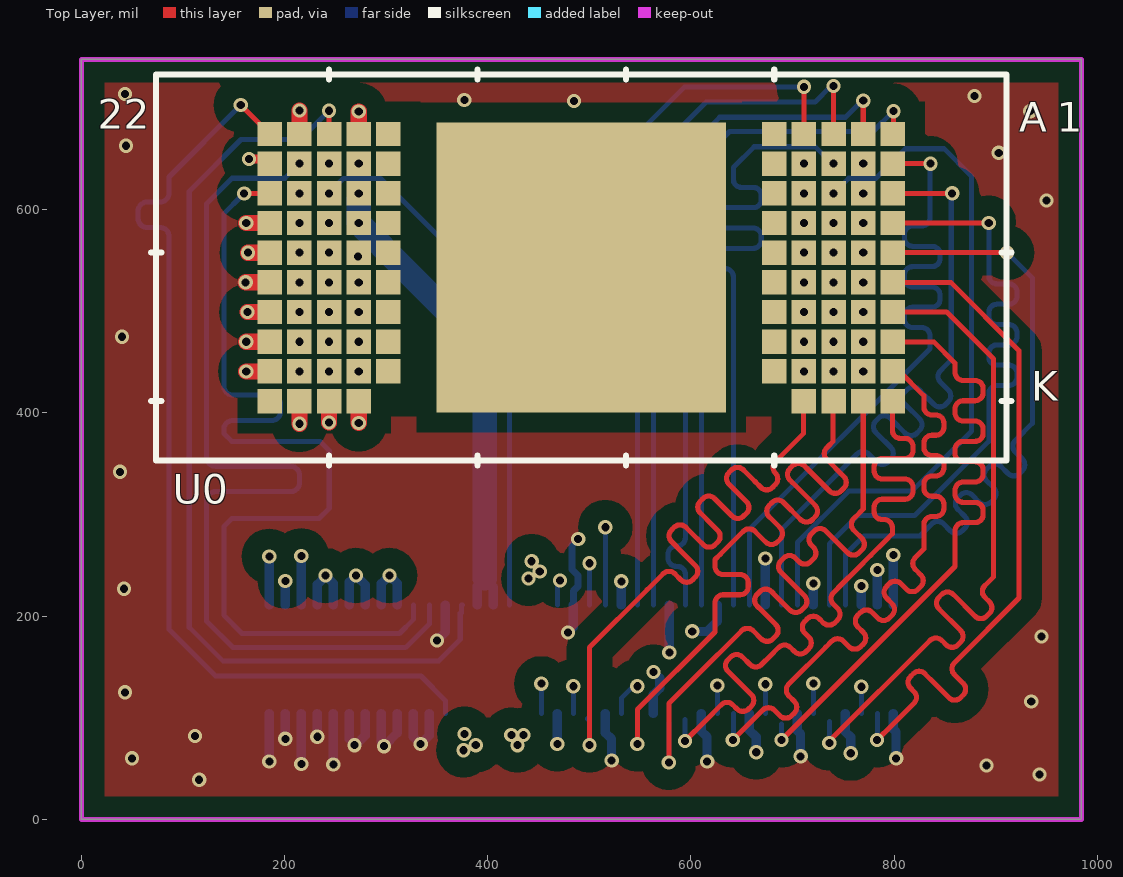
[diagram p0: Top Layer view]
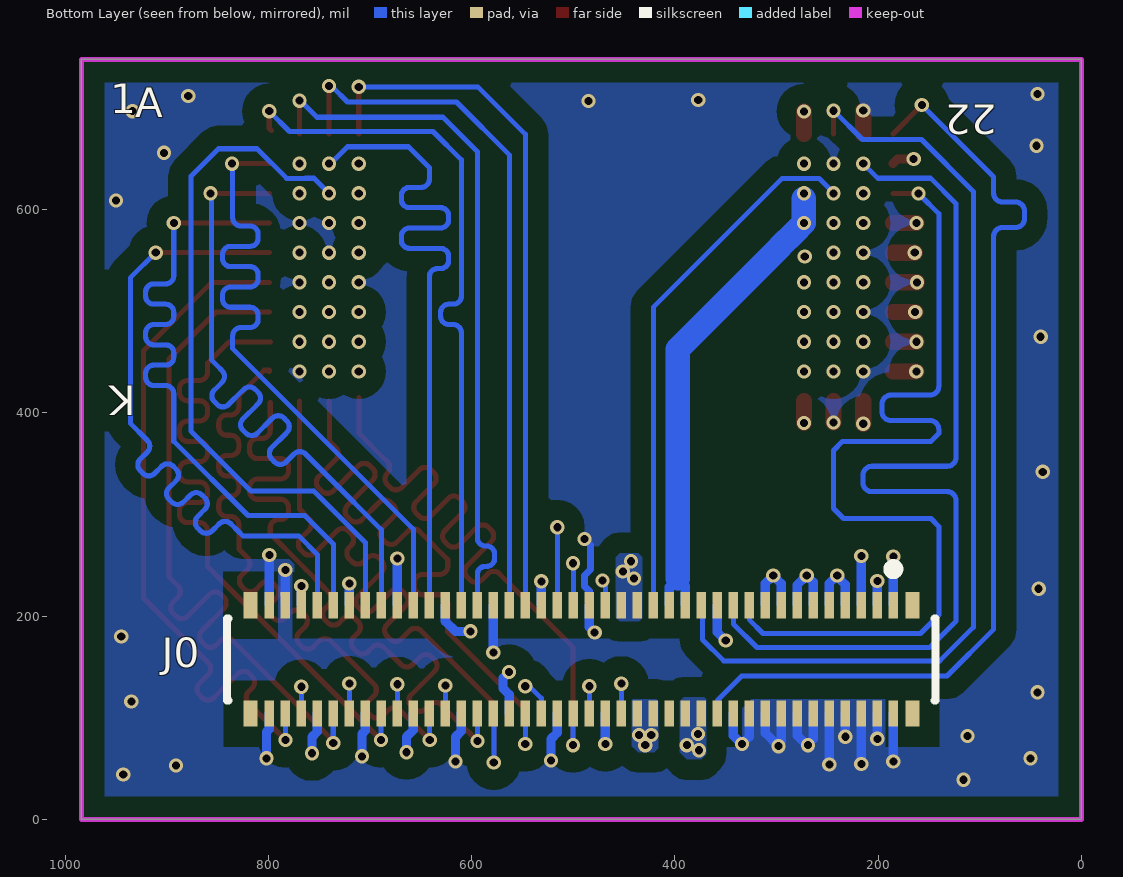
[diagram p1: Bottom Layer view, seen from below]
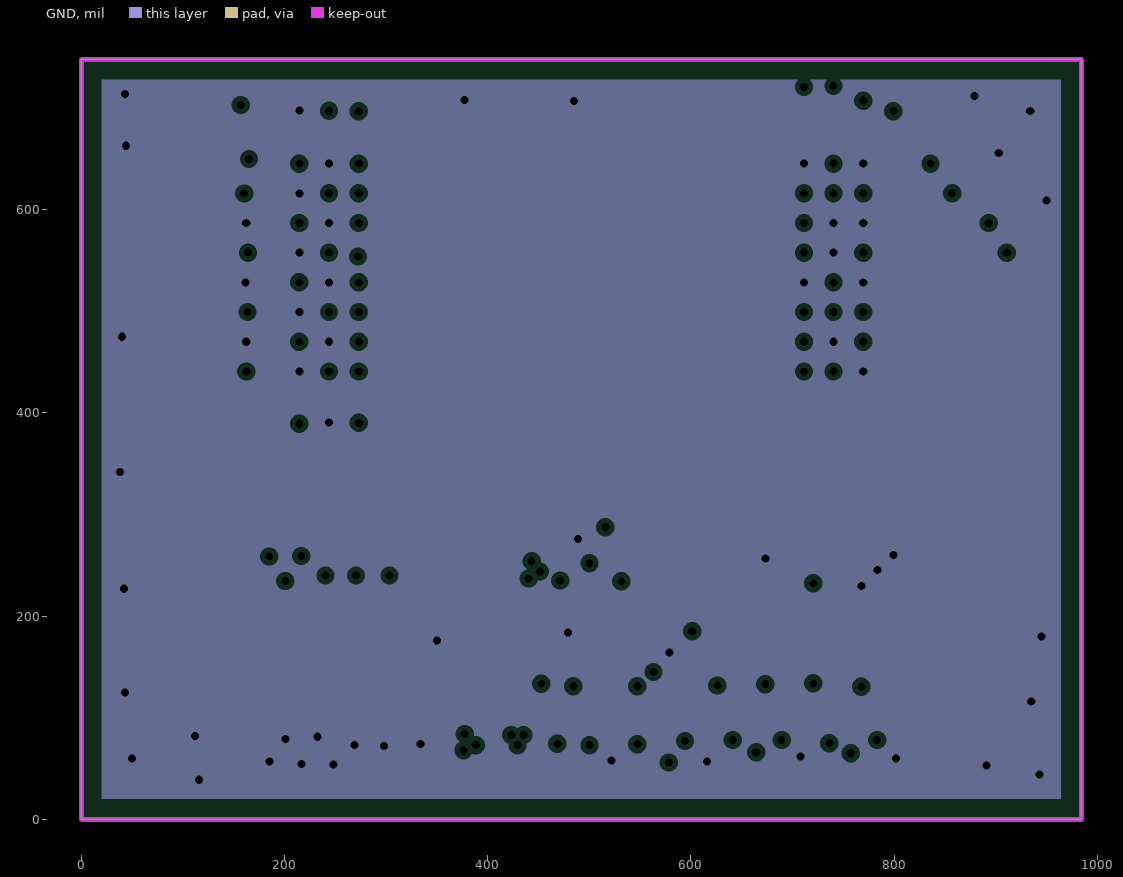
[diagram p2: GND, clearances drawn from the general rule]
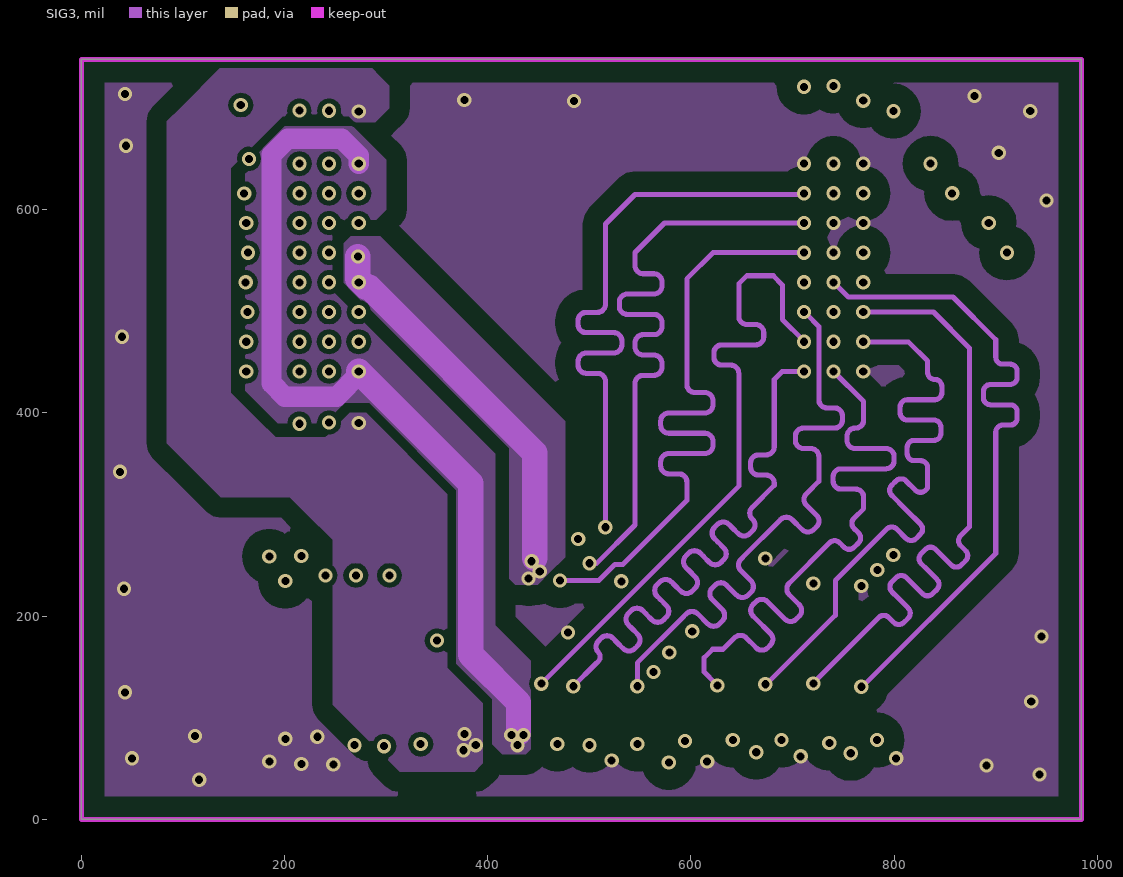
[diagram p3: SIG3]
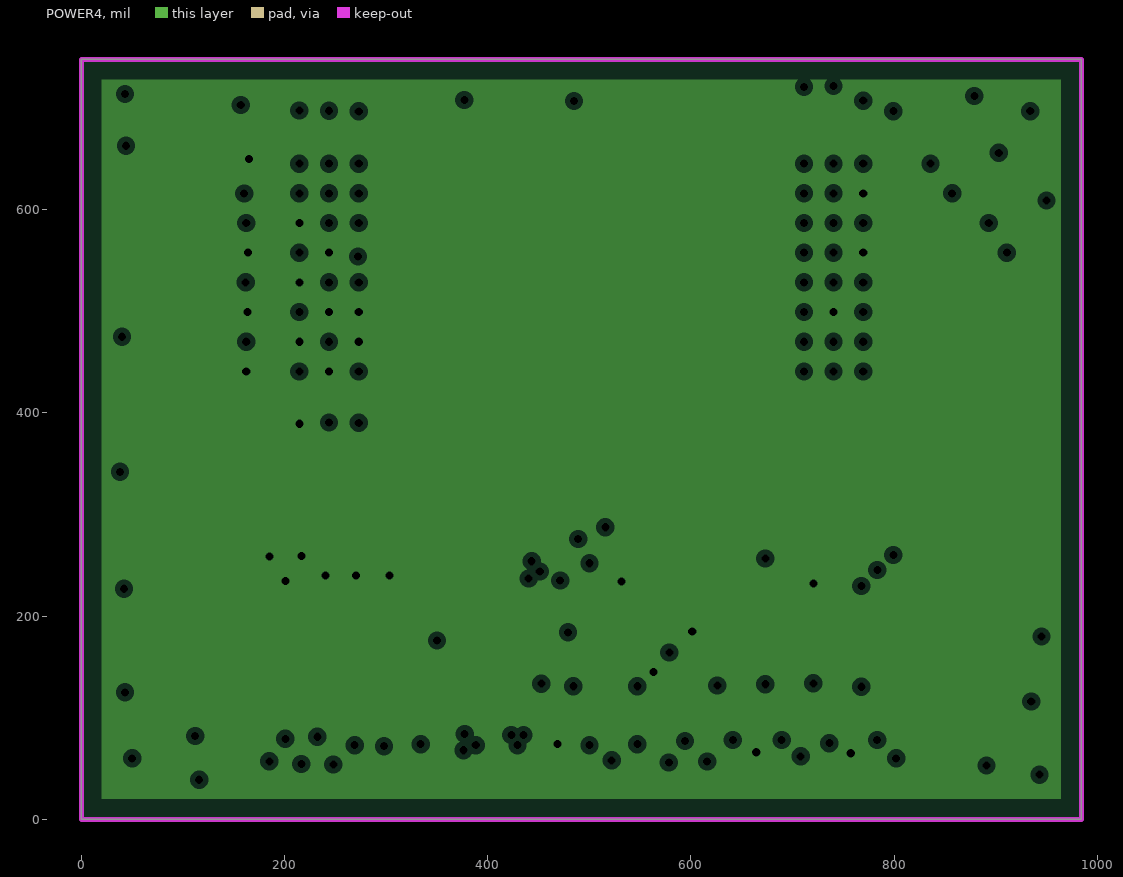
[diagram p4: POWER4, clearances drawn from the general rule]
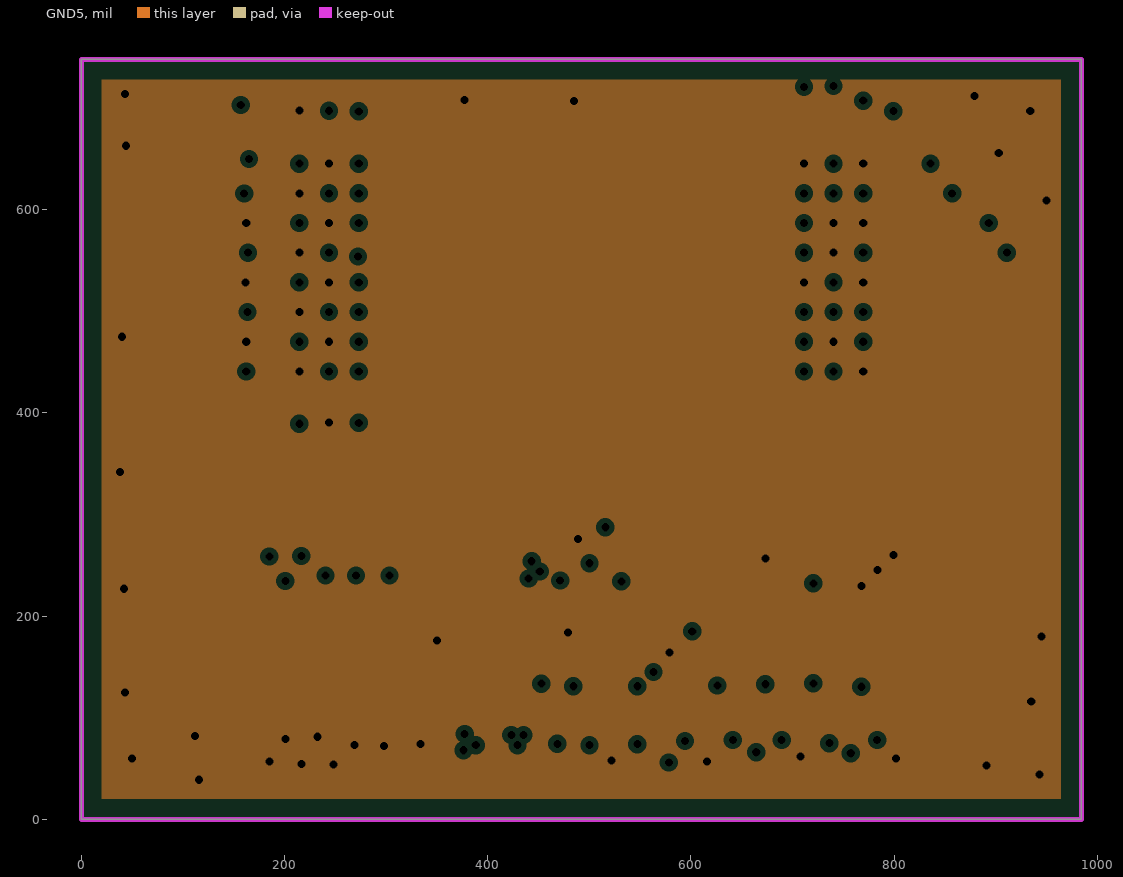
[diagram p5: GND5, clearances drawn from the general rule]
# Altium PCB MISC82783.PcbDoc
Units mil, origin at the board's own origin, x right, y up, seen from the top; angles counter-clockwise.
Board outline 984.25 x 748.03 mil, 6 copper layers (Top Layer, GND, SIG3, POWER4, GND5, Bottom Layer), stack 61.556 mil thick; 2 components, 40 nets, 183 pads, 150 vias.

## Layer stack, top to bottom
Top Layer: signal copper 1.378
Dielectric: core 2.8, PP-006, Dk 4.1
GND: plane copper 1.4, net GND
Dielectric: prepreg 12.6, FR-4, Dk 4.8
SIG3: signal copper 1.4
Dielectric: core 12.6, FR-4, Dk 4.8
POWER4: plane copper 1.4, net VCC
Dielectric: prepreg 12.6, FR-4, Dk 4.8
GND5: plane copper 1.4, net GND
Dielectric: core 12.6, FR-4, Dk 4.8
Bottom Layer: signal copper 1.378

## Board outline
0,0 984.25,0 984.25,748.03 0,748.03

## Design rules (kind name [scope] priority, off if disabled: settings)
Clearance Clearance_1 [inpolygon] p1: gap=5
Clearance [All] p2: gap=5
DiffPairsRouting [All] p1: maxlimit=5 minlimit=5 mostfreqgap=5 maxuncoupledlength=500
HoleSize [All] p1: absolutevalues=TRUE maxlimit=196.85 minlimit=1 maxpercent=80.000 minpercent=20.000
HoleToHoleClearance [All] p1: gap=0 allowstackedmicrovias=TRUE
MinimumSolderMaskSliver [All] p1: minsoldermaskwidth=0
PlaneClearance [All] p1: clearance=5
PlaneConnect [All] p1: planeconnectstyle=Direct reliefexpansion=20 reliefentries=4 reliefconductorwidth=10 reliefairgap=10
PolygonConnect [All] p1: connectstyle=Direct reliefconductorwidth=10 reliefentries=4 polygonreliefangle="90 Angle"
RoutingCorners [All] p1: cornerstyle=Round minsetback=100 maxsetback=100
RoutingVias [All] p1: holewidth=8 width=14 viastyle="Through Hole" minholewidth=8 minwidth=14 maxholewidth=8 maxwidth=14
SilkToSilkClearance [All] p1: silktosilkclearance=0
SilkscreenOverComponentPads SilkToSolderMaskClearance [IsPad] p1: minsilkscreentomaskgap=0
SolderMaskExpansion [All] p1: expansion=4
Width [All] p1: maxlimit=40 minlimit=5 preferedwidth=5
19 further rules are at their usual default settings.

## Components (designator, comment, footprint, x,y, rotation, side; value= is the part's Value field where it differs from the comment)
J0 "DF40C-80DP-0.4V_51" HIROSE_DF40C-80DP-0.4V_51_0 492.13,157.48 r0 bottom locked
U0 "DLP4500AFQD" LGA_0AFQD_TEX 492.13,543.11 r180 top locked

## Footprints (in the part's own frame and the unit in brackets; to place one, negate y for a bottom-side part, rotate by r counter-clockwise, add the part's x,y. Pads: shape width x height; smd on the part's side, far side on the other; paste and mask are expansions set on the pad)
HIROSE_DF40C-80DP-0.4V_51_0 [mm]
  rect 0.23x0.66 smd paste-1000 mask+0: 1(-7.8,-1.355) 2(-7.8,1.355) 3(-7.4,-1.355) 4(-7.4,1.355) 5(-7,-1.355) 6(-7,1.355) 7(-6.6,-1.355) 8(-6.6,1.355) 9(-6.2,-1.355) 10(-6.2,1.355) 11(-5.8,-1.355) 12(-5.8,1.355) 13(-5.4,-1.355) 14(-5.4,1.355) 15(-5,-1.355) 16(-5,1.355) 17(-4.6,-1.355) 18(-4.6,1.355) 19(-4.2,-1.355) 20(-4.2,1.355) 21(-3.8,-1.355) 22(-3.8,1.355) 23(-3.4,-1.355) 24(-3.4,1.355) 25(-3,-1.355) 26(-3,1.355) 27(-2.6,-1.355) 28(-2.6,1.355) 29(-2.2,-1.355) 30(-2.2,1.355) 31(-1.8,-1.355) 32(-1.8,1.355) 33(-1.4,-1.355) 34(-1.4,1.355) 35(-1,-1.355) 36(-1,1.355) 37(-0.6,-1.355) 38(-0.6,1.355) 39(-0.2,-1.355) 40(-0.2,1.355) 41(0.2,-1.355) 42(0.2,1.355) 43(0.6,-1.355) 44(0.6,1.355) 45(1,-1.355) 46(1,1.355) 47(1.4,-1.355) 48(1.4,1.355) 49(1.8,-1.355) 50(1.8,1.355) 51(2.2,-1.355) 52(2.2,1.355) 53(2.6,-1.355) 54(2.6,1.355) 55(3,-1.355) 56(3,1.355) 57(3.4,-1.355) 58(3.4,1.355) 59(3.8,-1.355) 60(3.8,1.355) 61(4.2,-1.355) 62(4.2,1.355) 63(4.6,-1.355) 64(4.6,1.355) 65(5,-1.355) 66(5,1.355) 67(5.4,-1.355) 68(5.4,1.355) 69(5.8,-1.355) 70(5.8,1.355) 71(6.2,-1.355) 72(6.2,1.355) 73(6.6,-1.355) 74(6.6,1.355) 75(7,-1.355) 76(7,1.355) 77(7.4,-1.355) 78(7.4,1.355) 79(7.8,-1.355) 80(7.8,1.355)
  rect 0.35x0.66 smd paste-1000 mask+0: 81(-8.275,1.355) 82(8.275,1.355) 83(-8.275,-1.355) 84(8.275,-1.355)
  silkscreen extent -8.86,-2.38 8.86,1.02, body extent -8.76,-1.49 8.76,1.48, height 1.14
LGA_0AFQD_TEX [mil]
  rect 285x285 smd paste-142 mask+0: 99(0,0)
  rect 24x24 smd paste+0 mask+0: A1(-306.7,-131.46) A2(-277.49,-131.46) A3(-248.28,-131.46) A4(-219.07,-131.46) A5(-189.86,-131.46) A18(189.86,-131.46) A19(219.07,-131.46) A20(248.29,-131.46) A21(277.49,-131.46) A22(306.7,-131.46) B1(-306.7,-102.24) B2(-277.49,-102.24) B3(-248.28,-102.24) B4(-219.07,-102.24) B5(-189.86,-102.24) B18(189.86,-102.24) B19(219.07,-102.24) B20(248.29,-102.24) B21(277.49,-102.24) B22(306.7,-102.24) C1(-306.7,-73.03) C2(-277.49,-73.03) C3(-248.28,-73.03) C4(-219.07,-73.03) C5(-189.86,-73.03) C18(189.86,-73.03) C19(219.07,-73.03) C20(248.29,-73.03) C21(277.49,-73.03) C22(306.7,-73.03) D1(-306.7,-43.82) D2(-277.49,-43.82) D3(-248.28,-43.82) D4(-219.07,-43.82) D5(-189.86,-43.82) D18(189.86,-43.82) D19(219.07,-43.82) D20(248.29,-43.82) D21(277.49,-43.82) D22(306.7,-43.82) E1(-306.7,-14.61) E2(-277.49,-14.61) E3(-248.28,-14.61) E4(-219.07,-14.61) E5(-189.86,-14.61) E18(189.86,-14.61) E19(219.07,-14.61) E20(248.29,-14.61) E21(277.49,-14.61) E22(306.7,-14.61) F1(-306.7,14.61) F2(-277.49,14.61) F3(-248.28,14.61) F4(-219.07,14.61) F5(-189.86,14.61) F18(189.86,14.61) F19(219.07,14.61) F20(248.29,14.61) F21(277.49,14.61) F22(306.7,14.61) G1(-306.7,43.82) G2(-277.49,43.82) G3(-248.28,43.82) G4(-219.07,43.82) G5(-189.86,43.82) G18(189.86,43.82) G19(219.07,43.82) G20(248.29,43.82) G21(277.49,43.82) G22(306.7,43.82) H1(-306.7,73.03) H2(-277.49,73.03) H3(-248.28,73.03) H4(-219.07,73.03) H5(-189.86,73.03) H18(189.86,73.03) H19(219.07,73.03) H20(248.29,73.03) H21(277.49,73.03) H22(306.7,73.03) J1(-306.7,102.24) J2(-277.49,102.24) J3(-248.28,102.24) J4(-219.07,102.24) J5(-189.86,102.24) J18(189.86,102.24) J19(219.07,102.24) J20(248.29,102.24) J21(277.49,102.24) J22(306.7,102.24) K1(-306.7,131.46) K2(-277.49,131.46) K3(-248.28,131.46) K4(-219.07,131.46) K19(219.07,131.46) K20(248.29,131.46) K21(277.49,131.46) K22(306.7,131.46)
  silkscreen extent -424,-195 424,195, body extent -414,-185 414,185, height 135

## Part data
U0: "No Description Available"

## Via types
v1: diameter 14, hole 8, Top Layer to Bottom Layer, 150 vias

## Nets (pads, with @x,y where several pads share a name; then routed paths per layer and width w, separated by ;. In a path a pad name is that pad's centre, name@x,y a point inside that pad or via, vN(x,y) a via of type N, cw(c..) or ccw(c..) an arc to the next point about the centre after c; other vN are vias at no path point)
DAD_BUS: J0.21 U0.B21 | length 945
  Bottom Layer w5: v1(214.63,645.35) 200.28,631 148.26,631 123.26,606 123.26,360 123.26,356.25 ccw(c132.01,356.25) 132.01,347.5 206.07,347.5 cw(c206.07,338.75) 214.82,338.75 214.82,331.25 cw(c206.07,331.25) 206.07,322.5 132.01,322.5 ccw(c132.01,313.75) 123.26,313.75 123.26,303 123.26,195 149.26,169 319.26,169 342.52,192.26 J0.21
DAD_OEZ: J0.25 U0.A20 | length 945.9
  Top Layer w5: U0.A20 v1(243.84,697.42)
  Bottom Layer w5: v1@243.26,697 215.26,669 157.26,669 106.26,618 106.26,189 139.26,156 352,156 373,177 J0.25@373,203 ; J0.25@374,203 J0.25@374,210 ; J0.25 J0.25@374.02,210.02 ; J0.25@375,211 J0.25@374.02,210.02
DAD_STRB: J0.24 U0.A22 | length 945
  Top Layer w5: v1(156.98,703.01) U0.A22
  Bottom Layer w5: v1(156.98,703.01) 86.26,632.29 86.26,629 86.26,616.25 cw(c77.51,616.25) 77.51,607.5 64.69,607.5 ccw(c64.69,598.75) 55.94,598.75 55.94,591.25 ccw(c64.69,591.25) 64.69,582.5 77.51,582.5 cw(c77.51,573.75) 86.26,573.75 86.26,570 86.26,187 132.26,141 334.26,141 358.27,116.99 J0.24
DATA0: J0.55 U0.A1 | length 694
  Top Layer w5: U0.A1@797.26,678 799.26,680 v1(799.26,697)
  Bottom Layer w5: J0.55 610.24,456 610.24,479 cw(c618.24,479) 618.24,487 622.58,487 ccw(c622.58,495) 630.58,495 630.58,499 ccw(c622.58,499) 622.58,507 618.24,507 cw(c618.24,515) 610.24,515 610.24,517 610.24,649.24 638,677 779.26,677 v1(799.26,697)
DATA1: J0.53 U0.A2 | length 694
  Top Layer w5: U0.A2 v1(769.62,707.36)
  Bottom Layer w5: J0.53 594.49,226 594.49,239 594.49,241 ccw(c586.49,241) 586.49,249 585.41,249 cw(c585.41,257) 577.41,257 577.41,261 cw(c585.41,261) 585.41,269 586.49,269 ccw(c586.49,277) 594.49,277 594.49,307 594.49,657.23 628.26,691 752.26,691 v1@768.26,707
DATA2: J0.49 U0.A3 | length 694.9
  Top Layer w5: U0.A3 v1(740.41,721.85)
  Bottom Layer w5: J0.49 562.99,653.99 615,706 722.26,706 v1@737.26,721 ; v1@738.26,721 v1@737.26,721 ; v1@738.26,722 v1@737.26,721
DATA3: J0.47 U0.A4 | length 693.1
  Top Layer w5: U0.A4 v1(711.2,720.94)
  Bottom Layer w5: J0.47 547.24,674.24 593.94,720.94 v1(711.2,720.94)
DATA4: J0.61 U0.B1 | length 694
  Top Layer w5: U0.B1 v1(835.91,645.35)
  Bottom Layer w5: J0.61 657.48,285.48 835.26,463.26 835.26,474 835.26,476 ccw(c827.26,476) 827.26,484 818.21,484 cw(c818.21,492) 810.21,492 810.21,496 cw(c818.21,496) 818.21,504 835.26,504 837.26,504 ccw(c837.26,512) 845.26,512 845.26,516 ccw(c837.26,516) 837.26,524 835.26,524 818.21,524 cw(c818.21,532) 810.21,532 810.21,536 cw(c818.21,536) 818.21,544 835.26,544 837.26,544 ccw(c837.26,552) 845.26,552 845.26,556 ccw(c837.26,556) 837.26,564 835.26,564 818.21,564 cw(c818.21,572) 810.21,572 810.21,576 cw(c818.21,576) 818.21,584 827.26,584 ccw(c827.26,592) 835.26,592 835.26,620 v1@835.26,645
DATA5: J0.59 U0.B3 | length 694
  Bottom Layer w5: J0.59 641.73,500 641.73,534 ccw(c633.73,534) 633.73,542 630.73,542 cw(c630.73,550) 622.73,550 622.73,554 cw(c630.73,554) 630.73,562 641.73,562 661.24,562 ccw(c661.24,570) 669.24,570 669.24,574 ccw(c661.24,574) 661.24,582 641.73,582 630.73,582 cw(c630.73,590) 622.73,590 622.73,594 cw(c630.73,594) 630.73,602 641.73,602 661.24,602 ccw(c661.24,610) 669.24,610 669.24,614 ccw(c661.24,614) 661.24,622 649.73,622 cw(c649.73,630) 641.73,630 641.73,632 641.73,641.47 662.26,662 722.26,662 v1@738.26,646
  other v1: 740.41,645.35
DATA6: J0.65 U0.C1 | length 694
  Top Layer w5: U0.C1 v1(857.12,616.14)
  Bottom Layer w5: J0.65 688.98,284.98 741.5,337.5 763.56,359.56 cw(c769.22,353.9) 774.88,359.56 782.71,351.73 ccw(c788.36,357.39) 794.02,351.73 796.85,354.56 ccw(c791.19,360.22) 796.85,365.87 783.36,379.36 781.95,380.77 cw(c787.6,386.43) 781.95,392.09 784.77,394.92 cw(c790.43,389.26) 796.09,394.92 797.5,393.5 810.99,380.01 ccw(c816.65,385.67) 822.3,380.01 825.13,382.84 ccw(c819.48,388.5) 825.13,394.16 811.64,407.64 810.23,409.06 cw(c815.89,414.72) 810.23,420.37 813.06,423.2 cw(c818.72,417.54) 824.37,423.2 825.79,421.79 839.27,408.3 ccw(c844.93,413.96) 850.59,408.3 853.42,411.13 ccw(c847.76,416.78) 853.42,422.44 845.59,430.27 cw(c851.24,435.93) 845.59,441.59 847,443 856.26,452.26 v1@856.26,616
DATA7: J0.67 U0.C3 | length 694.9
  Bottom Layer w5: J0.67 704.72,272.46 755.26,323 817.26,323 876.26,382 876.26,633 849.26,660 811.26,660 782.11,630.85 763.61,630.85 763.47,631 755.27,631 v1(740.41,616.14)
DATA8: J0.43 U0.C4 | length 694
  SIG3 w5: v1(515.75,287.49) 516,287.74 516,429 516,431 ccw(c508,431) 508,439 497.01,439 cw(c497.01,447) 489.01,447 489.01,451 cw(c497.01,451) 497.01,459 516,459 523.99,459 ccw(c523.99,467) 531.99,467 531.99,471 ccw(c523.99,471) 523.99,479 516,479 497.01,479 cw(c497.01,487) 489.01,487 489.01,491 cw(c497.01,491) 497.01,499 508,499 ccw(c508,507) 516,507 516,559 516,586 545,615 v1@710.26,615
  Bottom Layer w5: J0.43 v1(515.75,287.49)
  other v1: 711.2,616.14
DATA9: J0.71 U0.D1 | length 694
  Top Layer w5: U0.D1 v1(893.19,586.93)
  Bottom Layer w5: J0.71 736.22,270.96 764.26,299 820.26,299 893.26,372 893.26,419 cw(c901.26,419) 901.26,427 912.9,427 ccw(c912.9,435) 920.9,435 920.9,439 ccw(c912.9,439) 912.9,447 901.26,447 cw(c901.26,455) 893.26,455 893.26,459 cw(c901.26,459) 901.26,467 912.9,467 ccw(c912.9,475) 920.9,475 920.9,479 ccw(c912.9,479) 912.9,487 901.26,487 cw(c901.26,495) 893.26,495 893.26,499 cw(c901.26,499) 901.26,507 912.9,507 ccw(c912.9,515) 920.9,515 920.9,519 ccw(c912.9,519) 912.9,527 901.26,527 cw(c901.26,535) 893.26,535 v1@893.26,588
DATA10: J0.41 U0.D4 | length 694
  SIG3 w5: v1(500.26,252) 507.26,252 545,289.74 545,376 545,429 cw(c553,429) 553,437 563.49,437 ccw(c563.49,445) 571.49,445 571.49,449 ccw(c563.49,449) 563.49,457 553,457 cw(c553,465) 545,465 545,469 cw(c553,469) 553,477 563.49,477 ccw(c563.49,485) 571.49,485 571.49,489 ccw(c563.49,489) 563.49,497 545,497 537.5,497 cw(c537.5,505) 529.5,505 529.5,509 cw(c537.5,509) 537.5,517 545,517 563.49,517 ccw(c563.49,525) 571.49,525 571.49,529 ccw(c563.49,529) 563.49,537 553,537 cw(c553,545) 545,545 545,547 545,558 573.93,586.93 v1(711.2,586.93)
  Bottom Layer w5: J0.41 v1@500,249.26
DATA11: J0.73 U0.E1 | length 694
  Top Layer w5: U0.E1 v1(910.98,557.72)
  Bottom Layer w5: J0.73 751.97,260.71 770.26,279 825.26,279 829.63,283.37 837.19,290.93 cw(c842.85,285.27) 848.51,290.93 855.57,283.87 ccw(c861.22,289.53) 866.88,283.87 869.71,286.7 ccw(c864.05,292.36) 869.71,298.01 862.65,305.07 cw(c868.3,310.73) 862.65,316.39 865.48,319.22 cw(c871.13,313.56) 876.79,319.22 883.85,312.16 ccw(c889.51,317.81) 895.16,312.16 897.99,314.98 ccw(c892.33,320.64) 897.99,326.3 890.93,333.36 cw(c896.59,339.01) 890.93,344.67 893.76,347.5 cw(c899.42,341.84) 905.07,347.5 912.13,340.44 ccw(c917.79,346.1) 923.45,340.44 926.28,343.27 ccw(c920.62,348.93) 926.28,354.58 919.22,361.64 cw(c924.87,367.3) 919.22,372.96 920.63,374.37 936,389.74 936,532.98 v1@911.26,557.72 ; v1@911.26,558 v1@911.26,557.72 ; v1@911.26,559 v1@911.26,557.72
DATA12: J0.37 U0.E4 | length 694
  SIG3 w5: v1(471.26,235) 509.26,235 525.26,251 533.26,251 596,313.74 596,330 596,332 ccw(c588,332) 588,340 578.26,340 cw(c578.26,348) 570.26,348 570.26,352 cw(c578.26,352) 578.26,360 596,360 613.74,360 ccw(c613.74,368) 621.74,368 621.74,372 ccw(c613.74,372) 613.74,380 596,380 578.26,380 cw(c578.26,388) 570.26,388 570.26,392 cw(c578.26,392) 578.26,400 596,400 613.74,400 ccw(c613.74,408) 621.74,408 621.74,412 ccw(c613.74,412) 613.74,420 604,420 cw(c604,428) 596,428 596,462 596,532 621.72,557.72 v1(711.2,557.72)
  Bottom Layer w5: J0.37 v1@468.5,231.76
DATA13: J0.78 U0.F1 | length 694
  Top Layer w5: v1(783.26,78) 797.63,92.37 819.62,114.36 ccw(c813.96,120.01) 819.62,125.67 816.05,129.23 cw(c821.71,134.89) 816.05,140.55 818.88,143.38 cw(c824.54,137.72) 830.2,143.38 839.42,134.16 853.92,119.65 ccw(c859.58,125.31) 865.23,119.65 868.06,122.48 ccw(c862.4,128.14) 868.06,133.8 859.22,142.64 cw(c864.87,148.3) 859.22,153.96 860.63,155.37 923,217.74 923,461.26 855.76,528.5 U0.F1
  Bottom Layer w5: v1@783.46,81.8 J0.78
DATA14: J0.76 U0.F3 | length 694
  SIG3 w5: v1(740.41,528.5) 754.91,514 858,514 900,472 900,458 900,455 ccw(c907,455) 907,448 914.12,448 cw(c914.12,441) 921.12,441 921.12,435 cw(c914.12,435) 914.12,428 900,428 894.88,428 ccw(c894.88,421) 887.88,421 887.88,415 ccw(c894.88,415) 894.88,408 900,408 914.12,408 cw(c914.12,401) 921.12,401 921.12,395 cw(c914.12,395) 914.12,388 907,388 ccw(c907,381) 900,381 900,312 900,261.74 767.26,129 v1@765.26,129
  Bottom Layer w5: J0.76 v1(767.72,130.46)
DATA15: J0.72 U0.G1 | length 694.3
  Top Layer w5: v1(736.26,75) v1@737.26,76 ; v1@736.26,77 835.48,176.22 cw(c841.13,170.56) 846.79,176.22 851.41,171.6 ccw(c857.06,177.26) 862.72,171.6 865.55,174.43 ccw(c859.89,180.08) 865.55,185.74 844,207.29 cw(c849.66,212.94) 844,218.6 846.83,221.43 cw(c852.49,215.77) 858.14,221.43 879.69,199.88 ccw(c885.35,205.54) 891,199.88 893.83,202.71 ccw(c888.18,208.37) 893.83,214.03 889.22,218.64 cw(c894.87,224.3) 889.22,229.96 898,238.74 898,453 851.71,499.29 U0.G1
  Bottom Layer w5: v1(736.26,75) J0.72@736.26,96
DATA16: J0.70 U0.G2 | length 694
  SIG3 w5: v1@719.26,134 720.26,134 733.63,147.37 784.9,198.64 cw(c789.85,193.69) 794.8,198.64 799.69,193.75 ccw(c804.64,198.7) 809.59,193.75 813.83,197.99 ccw(c808.88,202.94) 813.83,207.89 803.99,217.73 797.89,223.83 cw(c802.84,228.78) 797.89,233.73 802.13,237.98 cw(c807.08,233.03) 812.03,237.98 818.13,231.87 827.97,222.03 ccw(c832.92,226.98) 837.87,222.03 842.12,226.27 ccw(c837.17,231.22) 842.12,236.17 832.27,246.01 826.64,251.65 cw(c831.59,256.6) 826.64,261.55 830.88,265.79 cw(c835.83,260.84) 840.78,265.79 846.42,260.16 856.26,250.31 ccw(c861.21,255.26) 866.16,250.31 870.4,254.56 ccw(c865.45,259.51) 870.4,264.46 865.51,269.35 cw(c870.46,274.3) 865.51,279.25 867.63,281.37 874,287.74 874,464 838.71,499.29 v1(769.62,499.29)
  Bottom Layer w5: J0.70 v1(720.47,133.79)
DATA17: J0.46 U0.G4 | length 694
  SIG3 w5: v1@547.26,132 547.26,154 591.13,197.87 595.48,202.22 cw(c601.13,196.56) 606.79,202.22 616.69,192.32 ccw(c622.35,197.97) 628,192.32 630.83,195.14 ccw(c625.17,200.8) 630.83,206.46 620.93,216.36 cw(c626.59,222.01) 620.93,227.67 623.76,230.5 cw(c629.42,224.84) 635.07,230.5 644.97,220.6 ccw(c650.63,226.26) 656.29,220.6 659.12,223.43 ccw(c653.46,229.09) 659.12,234.74 649.22,244.64 cw(c654.87,250.3) 649.22,255.96 650.63,257.37 688.13,294.87 688.26,295 cw(c693.92,289.34) 699.57,295 709.47,285.1 ccw(c715.13,290.76) 720.79,285.1 723.62,287.93 ccw(c717.96,293.59) 723.62,299.24 713.72,309.14 cw(c719.37,314.8) 713.72,320.46 715.13,321.87 725.91,332.65 725.91,355 725.91,357 ccw(c717.91,357) 717.91,365 710.78,365 cw(c710.78,373) 702.78,373 702.78,377 cw(c710.78,377) 710.78,385 725.91,385 741.04,385 ccw(c741.04,393) 749.04,393 749.04,397 ccw(c741.04,397) 741.04,405 733.91,405 cw(c733.91,413) 725.91,413 725.91,418 725.91,476.08 725.91,485.09 v1@714,497 ; v1(711.2,499.29) v1@713.75,496.75
  Bottom Layer w5: J0.46 531.5,119.24 543.26,131 v1(547.26,131)
DATA18: J0.66 U0.H1 | length 694
  Top Layer w5: v1(689.26,78) 860,248.74 860,284 cw(c868,284) 868,292 879.6,292 ccw(c879.6,300) 887.6,300 887.6,304 ccw(c879.6,304) 879.6,312 868,312 cw(c868,320) 860,320 860,324 cw(c868,324) 868,332 879.6,332 ccw(c879.6,340) 887.6,340 887.6,344 ccw(c879.6,344) 879.6,352 868,352 cw(c868,360) 860,360 860,364 cw(c868,364) 868,372 879.6,372 ccw(c879.6,380) 887.6,380 887.6,384 ccw(c879.6,384) 879.6,392 868,392 cw(c868,400) 860,400 860,404 cw(c868,404) 868,412 879.6,412 ccw(c879.6,420) 887.6,420 887.6,424 ccw(c879.6,424) 879.6,432 868,432 cw(c868,440) 860,440 860,442 860,449 839,470 U0.H1@798.26,470
  Bottom Layer w5: v1(689.26,78) J0.66@689.26,94
DATA19: J0.64 U0.H2 | length 694
  SIG3 w5: v1@673.26,132 742.13,200.87 742.13,235.13 778,271 792.69,285.69 cw(c797.64,280.75) 802.59,285.69 811.8,276.49 ccw(c816.75,281.44) 821.7,276.49 825.94,280.73 ccw(c820.99,285.68) 825.94,290.63 811.79,304.79 797.63,318.94 cw(c802.58,323.89) 797.63,328.84 801.87,333.08 cw(c806.82,328.13) 811.77,333.08 820.98,323.88 ccw(c825.93,328.83) 830.88,323.88 833,326 833,333 833,346 ccw(c826,346) 826,353 819.8,353 cw(c819.8,360) 812.8,360 812.8,366 cw(c819.8,366) 819.8,373 833,373 839.02,373 ccw(c839.02,380) 846.02,380 846.02,386 ccw(c839.02,386) 839.02,393 833,393 812.98,393 cw(c812.98,400) 805.98,400 805.98,406 cw(c812.98,406) 812.98,413 833,413 840,413 ccw(c840,420) 847,420 847,426 ccw(c840,426) 840,433 cw(c840,440) 833,440 833,443 833,451 814,470 v1@772,470 ; v1(769.62,470.08) v1@772.26,470.08
  Bottom Layer w5: J0.64 v1(673.23,132.97)
DATA20: J0.36 U0.H4 | length 694
  SIG3 w5: v1@453.26,134 647.13,327.87 647.13,437 647.13,439 ccw(c639.13,439) 639.13,447 630.57,447 cw(c630.57,455) 622.57,455 622.57,459 cw(c630.57,459) 630.57,467 647.13,467 663.69,467 ccw(c663.69,475) 671.69,475 671.69,479 ccw(c663.69,479) 663.69,487 655.13,487 cw(c655.13,495) 647.13,495 647.13,516 647.13,527.13 655,535 681,535 690,526 690,492 v1@711,471
  Bottom Layer w5: J0.36 v1(452.76,133.5)
  other v1: 711.2,470.08
DATA21: J0.60 U0.J1 | length 694
  Top Layer w5: v1(641.26,78) 664.63,101.37 670.76,107.5 cw(c676.42,101.84) 682.07,107.5 687.69,101.88 ccw(c693.35,107.54) 699,101.88 701.83,104.71 ccw(c696.18,110.37) 701.83,116.03 696.22,121.64 cw(c701.87,127.3) 696.22,132.96 697.63,134.37 732.63,169.37 738.69,175.43 cw(c744.35,169.77) 750.01,175.43 755.62,169.82 ccw(c761.28,175.47) 766.93,169.82 769.76,172.64 ccw(c764.11,178.3) 769.76,183.96 764.15,189.57 cw(c769.8,195.23) 764.15,200.89 766.98,203.72 cw(c772.63,198.06) 778.29,203.72 783.91,198.1 ccw(c789.56,203.76) 795.22,198.1 798.05,200.93 ccw(c792.39,206.58) 798.05,212.24 792.43,217.86 cw(c798.09,223.51) 792.43,229.17 795.26,232 cw(c800.92,226.34) 806.57,232 812.19,226.38 ccw(c817.85,232.04) 823.5,226.38 826.33,229.21 ccw(c820.68,234.87) 826.33,240.53 820.72,246.14 cw(c826.37,251.8) 820.72,257.46 822.13,258.87 829.26,266 829.26,280 829.26,290 cw(c837.26,290) 837.26,298 840.98,298 ccw(c840.98,306) 848.98,306 848.98,310 ccw(c840.98,310) 840.98,318 837.26,318 cw(c837.26,326) 829.26,326 829.26,330 cw(c837.26,330) 837.26,338 840.98,338 ccw(c840.98,346) 848.98,346 848.98,350 ccw(c840.98,350) 840.98,358 837.26,358 cw(c837.26,366) 829.26,366 829.26,370 cw(c837.26,370) 837.26,378 840.98,378 ccw(c840.98,386) 848.98,386 848.98,390 ccw(c840.98,390) 840.98,398 837.26,398 cw(c837.26,406) 829.26,406 829.26,408 829.26,417 804.26,442 U0.J1@799.26,442 ; U0.J1 U0.J1@799.26,440.87
  Bottom Layer w5: v1@641.73,81.53 J0.60
DATA22: J0.58 U0.J3 | length 694.1
  SIG3 w5: v1@624,132 624,134 613,145 613,159 621.37,167.37 631.63,167.37 642.98,178.72 cw(c648.63,173.06) 654.29,178.72 664.19,168.82 ccw(c669.85,174.47) 675.5,168.81 678.33,171.64 ccw(c672.67,177.3) 678.33,182.96 662.77,198.51 661.21,200.07 cw(c666.87,205.73) 661.21,211.38 ; v1@625.26,132 v1@625.98,132.72 ; v1@625.35,133.35 v1@625.98,132.72 ; v1(625.98,131.72) v1@625.98,132.72 ; 661.21,211.39 664.04,214.22 ; 664.05,214.22 cw(c669.7,208.56) 675.36,214.22 676.92,212.66 692.47,197.1 ccw(c698.13,202.76) 703.79,197.1 706.62,199.93 ; 706.62,199.94 ccw(c700.96,205.59) 706.62,211.24 696.72,221.14 cw(c702.37,226.8) 696.71,232.45 736.47,272.21 cw(c741.42,267.26) 746.37,272.21 750.77,267.81 ccw(c755.72,272.76) 760.67,267.81 764.91,272.05 ccw(c759.96,277) 764.91,281.95 760.51,286.35 cw(c765.46,291.3) 760.51,296.25 770,305.74 770,317 ccw(c762,317) 762,325 748,325 cw(c748,333) 740,333 740,337 cw(c748,337) 748,345 792,345 ccw(c792,353) 800,353 800,357 ccw(c792,357) 792,365 761.54,365 cw(c761.54,373) 753.54,373 753.54,377 cw(c761.54,377) 761.54,385 762,385 ccw(c762,393) 770,393 770,411.28 v1(740.41,440.87)
  Bottom Layer w5: J0.58 v1(625.98,131.72)
DATA23: J0.40 U0.J4 | length 694
  SIG3 w5: v1(484.25,130.99) 506.13,152.87 508.93,155.67 ccw(c504.65,159.94) 508.93,164.21 cw(c514.58,169.87) 508.93,175.53 511.76,178.36 cw(c517.41,172.7) 523.07,178.36 527.34,174.08 533.42,168.01 ccw(c539.08,173.66) 544.73,168.01 547.56,170.83 ccw(c541.91,176.49) 547.56,182.15 541.49,188.23 538.41,191.3 cw(c544.06,196.96) 538.41,202.62 541.24,205.45 cw(c546.89,199.79) 552.55,205.44 555.63,202.37 561.7,196.29 ccw(c567.36,201.95) 573.02,196.29 575.85,199.12 ccw(c570.19,204.78) 575.85,210.43 569.77,216.51 566.69,219.59 cw(c572.35,225.24) 566.69,230.9 569.52,233.73 cw(c575.18,228.07) 580.83,233.73 583.91,230.65 589.99,224.57 ccw(c595.65,230.23) 601.3,224.57 604.13,227.4 ccw(c598.47,233.06) 604.13,238.72 598.05,244.79 594.98,247.87 cw(c600.63,253.53) 594.98,259.19 597.8,262.01 cw(c603.46,256.36) 609.12,262.01 612.2,258.94 618.27,252.86 ccw(c623.93,258.52) 629.59,252.86 632.42,255.69 ccw(c626.76,261.34) 632.42,267 626.34,273.08 623.26,276.16 cw(c628.92,281.81) 623.26,287.47 626.09,290.3 cw(c631.75,284.64) 637.4,290.3 640.48,287.22 646.56,281.14 ccw(c652.21,286.8) 657.87,281.14 660.7,283.97 ccw(c655.04,289.63) 660.7,295.29 660.28,295.71 cw(c665.94,301.36) 660.28,307.02 682,328.74 682,330.74 ccw(c674,330.74) 674,338.74 666.82,338.74 cw(c666.82,346.74) 658.82,346.74 658.82,350.74 cw(c666.82,350.74) 666.82,358.74 674,358.74 ccw(c674,366.74) 682,366.74 682,403 682,433 689.87,440.87 v1(711.2,440.87)
  Bottom Layer w5: J0.40 v1(484.25,130.99)
DCLK: J0.54 U0.K1 | length 694
  Top Layer w5: v1@594,77 v1(594.26,77) 614.63,97.37 629.97,112.71 cw(c635.63,107.05) 641.28,112.71 645.41,108.58 ccw(c651.07,114.24) 656.72,108.58 659.55,111.41 ccw(c653.9,117.07) 659.55,122.72 649.77,132.51 636.48,145.79 cw(c642.14,151.45) 636.48,157.11 639.31,159.93 cw(c644.97,154.28) 650.62,159.93 658.25,152.31 ccw(c663.91,157.96) 669.57,152.31 678.05,160.79 686.54,169.28 cw(c692.19,163.62) 697.85,169.28 701.98,165.15 ccw(c707.64,170.81) 713.29,165.15 716.12,167.98 ccw(c710.46,173.63) 716.12,179.29 711.99,183.42 cw(c717.65,189.08) 711.99,194.73 714.82,197.56 cw(c720.48,191.9) 726.13,197.56 730.26,193.43 ccw(c735.92,199.09) 741.58,193.43 744.41,196.26 ccw(c738.75,201.92) 744.41,207.58 740.28,211.7 cw(c745.93,217.36) 740.28,223.02 748.76,231.5 762.9,245.64 777.05,259.79 791.19,273.93 798.26,281 798.26,287 ccw(c790.26,287) 790.26,295 788.31,295 cw(c788.31,303) 780.31,303 780.31,307 cw(c788.31,307) 788.31,315 798.26,315 810.57,315 ccw(c810.57,323) 818.57,323 818.57,327 ccw(c810.57,327) 810.57,335 798.26,335 788.31,335 cw(c788.31,343) 780.31,343 780.31,347 cw(c788.31,347) 788.31,355 798.26,355 810.57,355 ccw(c810.57,363) 818.57,363 818.57,367 ccw(c810.57,367) 810.57,375 806.26,375 cw(c806.26,383) 798.26,383 798.26,385 U0.K1@798.26,410
  Bottom Layer w5: v1(594.26,77) J0.54@594.26,98
GND: J0.2 J0.4 J0.6 J0.8 J0.10 J0.12 J0.14 J0.16 J0.18 J0.20 J0.22 J0.23 J0.39 J0.44 J0.51 J0.56 J0.63 J0.68 J0.75 J0.77 J0.79 J0.80 U0.A21 U0.B2 U0.B4 U0.B20 U0.C21 U0.D2 U0.D3 U0.D20 U0.D22 U0.E3 U0.E21 U0.F2 U0.F4 U0.F20 U0.F22 U0.G21 U0.H3 U0.H20 U0.H22 U0.J2 U0.J21 U0.K20 | length 1029
  Top Layer w16: v1(161.76,528.5) U0.F22 ; v1(162.34,470.08) U0.H22 ; v1(162.33,586.93) U0.D22 ; U0.A21 v1(214.63,697.63) ; v1(243.84,390.58) U0.K20
  Bottom Layer w7: J0.39 484.25,224.62 489,229.37 489,240 483,246 483,270 v1(489,276)
  Bottom Layer w9: v1(185.04,57.04) J0.2 ; v1(200.79,79.21) J0.4 ; v1(216.54,54.54) J0.6 ; v1(232.28,81.28) J0.8 ; v1(248.03,54.03) J0.10 ; J0.12 263.78,79.22 269,74 v1(269,73) ; v1@270,73 279.53,82.53 J0.14 ; v1@295.28,76.72 J0.16 ; v1(298,72) 311.02,85.02 J0.18 ; J0.20 326.77,81.23 v1@333,75 ; v1(334,74) 342.52,82.52 J0.22 ; v1(350,176) 358.27,184.27 358.27,185.27 J0.23 ; v1(479,184) 484.25,189.25 J0.39 ; J0.44 515.75,85.25 522,79 v1(522,58) ; v1(578.74,164.26) J0.51 ; J0.56 610.24,86.76 616,81 v1(616,57) ; J0.63 v1(673.23,256.77) ; J0.68 704.72,87.28 708,84 v1(708,62) ; J0.75 v1(767.72,229.72) ; J0.77 v1(783.46,245.46) ; J0.80 799.21,88.79 802,86 v1(802,60) ; J0.79 v1(799.21,260.21)
  other v1: 116,39 943,44 891,53 50,60 112,82 935,116 43,125 945,180 42,227 38,342 214.63,440.87 769.62,440.87 243.84,470.08 740.41,470.08 40,475 214.63,499.29 243.84,528.5 711.2,528.5 769.62,528.5 214.63,557.72 740.41,557.72 243.84,586.93 740.41,586.93 769.62,586.93 950,609 214.63,616.14 243.84,645.35 711.2,645.35 769.62,645.35 903,656 44,663 934,697 485,707 377,708 879,712 43,714
LOADB: J0.52 U0.K2 | length 693.2
  Top Layer w5: v1(578.26,56) 578.26,114 604.13,139.87 649.91,185.65 cw(c655.56,179.99) 661.22,185.65 669.34,177.53 ccw(c674.99,183.19) 680.65,177.53 683.48,180.36 ccw(c677.82,186.02) 683.48,191.67 669.71,205.45 665.1,210.06 cw(c670.75,215.71) 665.1,221.37 667.92,224.2 cw(c673.58,218.54) 679.24,224.2 683.85,219.59 697.62,205.82 ccw(c703.28,211.47) 708.94,205.82 711.76,208.64 ccw(c706.11,214.3) 711.76,219.96 697.99,233.73 688.6,243.12 cw(c694.26,248.78) 688.6,254.43 691.43,257.26 cw(c697.09,251.6) 702.74,257.26 706.48,253.53 ccw(c712.13,259.19) 717.79,253.53 720.62,256.36 ccw(c714.96,262.01) 720.62,267.67 718.59,269.7 cw(c724.25,275.36) 718.59,281.01 721.42,283.84 cw(c727.07,278.19) 732.73,283.84 740.42,276.16 754.19,262.38 ccw(c759.85,268.04) 765.5,262.38 768.33,265.21 ccw(c762.68,270.87) 768.33,276.53 760.22,284.64 cw(c765.87,290.3) 760.22,295.96 761.63,297.37 769.62,305.36 U0.K2
  Bottom Layer w5: v1(578.26,56) J0.52@578.26,95
SAC_BUS: J0.31 U0.C20 | length 528.5
  Bottom Layer w5: v1@244.26,617 258.11,630.85 294.41,630.85 421.26,504 J0.31
  other v1: 243.84,616.14
SAC_CLK: J0.19 U0.C22 | length 945
  Top Layer w5: v1@161.26,615 162.4,616.14 U0.C22
  Bottom Layer w5: v1@158.26,614 140.26,596 140.26,430 140.26,426.25 ccw(c149.01,426.25) 149.01,417.5 187.4,417.5 cw(c187.4,408.75) 196.15,408.75 196.15,401.25 cw(c187.4,401.25) 187.4,392.5 149.01,392.5 ccw(c149.01,383.75) 140.26,383.75 140.26,379.74 148,372 235,372 244,363 244,306 234,296 148,296 140.26,288.26 140.26,201 158.26,183 313.26,183 326.77,196.51 J0.19 ; v1@158.26,616 v1(160.26,616)
SCTRL: J0.48 U0.K3 | length 694
  Top Layer w5: v1(547.26,74) 547.26,108 623.63,184.37 623.63,205 623.63,213 cw(c631.63,213) 631.63,221 648.41,221 ccw(c648.41,229) 656.41,229 656.41,233 ccw(c648.41,233) 648.41,241 631.63,241 cw(c631.63,249) 623.63,249 623.63,251 623.63,255.63 628.93,260.93 643.08,275.08 651.56,283.56 cw(c657.22,277.9) 662.88,283.56 673.66,272.77 ccw(c679.32,278.43) 684.98,272.77 687.81,275.6 ccw(c682.15,281.26) 687.81,286.91 677.02,297.7 cw(c682.67,303.36) 677.02,309.02 679.85,311.85 cw(c685.5,306.19) 691.16,311.85 708.13,294.88 ccw(c713.79,300.53) 719.44,294.88 722.27,297.7 ccw(c716.62,303.36) 722.27,309.02 699.64,331.64 697.39,333.9 cw(c703.04,339.56) 697.39,345.22 700.22,348.04 cw(c705.87,342.39) 711.53,348.04 713.79,345.79 736.41,323.16 ccw(c742.07,328.82) 747.73,323.16 750.56,325.99 ccw(c744.9,331.64) 750.56,337.3 733.59,354.27 cw(c739.24,359.93) 733.59,365.59 735,367 740,372 U0.K3@740,409 ; U0.K3@740.41,409 U0.K3
  Bottom Layer w5: v1(547.26,74) J0.48@547.26,95
TEST_SCAN: J0.30
TRC: J0.42 U0.K4 | length 694
  Top Layer w5: v1(500.26,73) 500.26,169.26 557,226 572.78,241.78 cw(c578.43,236.12) 584.09,241.78 590.23,235.64 ccw(c595.89,241.3) 601.54,235.64 604.37,238.47 ccw(c598.71,244.12) 604.37,249.78 592.58,261.58 580.78,273.37 cw(c586.44,279.03) 580.78,284.68 583.61,287.51 cw(c589.27,281.86) 594.92,287.51 606.72,275.72 612.26,270.17 ccw(c617.92,275.83) 623.58,270.17 626.41,273 ccw(c620.75,278.66) 626.41,284.31 620.86,289.86 609.07,301.66 cw(c614.72,307.31) 609.07,312.97 611.89,315.8 cw(c617.55,310.14) 623.21,315.8 635,304 640.55,298.46 ccw(c646.21,304.11) 651.86,298.46 654.69,301.28 ccw(c649.03,306.94) 654.69,312.6 649.14,318.14 637.35,329.94 cw(c643.01,335.6) 637.35,341.25 640.18,344.08 cw(c645.84,338.42) 651.49,344.08 663.29,332.29 668.94,326.63 ccw(c674.6,332.29) 680.26,326.63 683.09,329.46 ccw(c677.43,335.12) 683.09,340.77 cw(c688.74,346.43) 683.09,352.09 684.5,353.5 711,380 U0.K4@711,415
  Bottom Layer w5: J0.42@498.26,99 500.26,97 v1(500.26,73)
VBIAS: J0.27 J0.29 U0.C19 U0.D19 | length 472.9
  Bottom Layer w9: J0.27 389.76,229.5 394.26,234 ; 402.26,232 405.51,228.75 J0.29
  Bottom Layer w24: v1@273.05,610.79 v1(273.05,586.93) 281.98,578 282.2,578 296.26,563.94 296.26,563.72 397.26,462.72 397.26,237
  other v1: 273.05,616.14
VCC: J0.1 J0.3 J0.5 J0.7 J0.9 J0.11 J0.13 J0.15 J0.17 J0.38 J0.45 J0.50 J0.57 J0.62 J0.69 J0.74 U0.B22 U0.C2 U0.D21 U0.E2 U0.E20 U0.E22 U0.F21 U0.G3 U0.G19 U0.G20 U0.G22 U0.H19 U0.H21 U0.J20 U0.J22 U0.K21 | length 666.6
  Top Layer w9: v1(165,650) 180.78,650 U0.B22
  Top Layer w16: v1(162.39,440.87) U0.J22 ; v1(163.55,499.29) U0.G22 ; v1(163.98,557.72) U0.E22 ; v1(214.63,389.37) U0.K21
  Bottom Layer w9: J0.1 v1(185.04,258.78) ; J0.3 v1(200.79,234.53) ; J0.5 v1(216.54,259.28) ; J0.7 232.28,231.02 v1@240.26,239 ; v1(240.26,240) 248.03,232.23 J0.9 ; J0.11 263.78,233.52 v1(270.26,240) ; v1@272.26,238 279.53,230.73 J0.13 ; J0.15 295.28,232.02 v1(303.26,240) ; v1@305.26,238 311.02,232.24 J0.17 ; v1(468.5,74.24) J0.38 ; J0.45 v1(531.5,234.24) ; J0.50 562.99,122.73 569.26,129 569.26,139 v1(563.26,145) ; v1(601.26,185) 616,185 625.98,194.98 J0.57 ; J0.62 657.48,87.78 664.26,81 v1(664.26,66) ; J0.69 v1(720.47,232.21) ; J0.74 751.97,86.29 757.26,81 v1(757.26,65)
  other v1: 243.84,440.87 214.63,470.08 273.05,470.08 243.84,499.29 273.05,499.29 740.41,499.29 214.63,528.5 243.84,557.72 769.62,557.72 214.63,586.93 769.62,616.14
VOFFSET: J0.26 J0.28 U0.A19 U0.K19 | length 43.7
  Top Layer w16: v1(273.05,390.21) U0.K19 ; U0.A19 v1(273.05,696.79)
  other v1: 376.26,68 388.26,73 377.26,84
VREF: J0.32 J0.34 U0.B19 U0.J19 | length 855.1
  SIG3 w20: v1(273.05,645.35) 273.05,653.21 256.26,670 203.26,670 187.26,654 187.26,429 200.26,416 251.26,416 v1@274.26,439
  SIG3 w25: v1(273.05,440.87) 383.26,330.66 383.26,162 430.26,115 v1@430.26,85
  other v1: 429.26,73 423.26,83 435.26,83
VRST: J0.33 J0.35 U0.E19 U0.F19 | length 370.7
  SIG3 w25: v1(272.26,554) 272.26,532 280.47,523.79 283.2,523.79 446.26,360.73 v1@446.26,257
  other v1: 440.26,237 451.26,244 443.26,254 273.05,528.5
pads on no net: J0.81 J0.82 J0.83 J0.84 U0.99 U0.A5 U0.A18 U0.B5 U0.B18 U0.C5 U0.C18 U0.D5 U0.D18 U0.E5 U0.E18 U0.F5 U0.F18 U0.G5 U0.G18 U0.H5 U0.H18 U0.J5 U0.J18 U0.K22

## Polygon pours and split planes (outlines as drawn)
GND on Bottom Layer "Bottom Layer-No Net" (solid, remove dead copper): -38,640 -38,0 -13,-25 4,-42 61,-42 1012,-42 1041,-13 1083,29 1083,65 1083,776 1050,809 1003,856 957,856 15,856 -19,822 -38,803 -38,642
VOFFSET on Bottom Layer "Bottom Layer-No Net" (solid, remove dead copper): 369.26,108 369.26,64 372.26,61 374.26,59 377.26,59 388.26,59 390.26,61 395.26,66 395.26,98 395.26,116 393.26,118 391.26,120 389.26,120 371.26,120 370.26,119 369.26,118 369.26,109
VRST on Bottom Layer "Bottom Layer-No Net" (solid, remove dead copper): 432.26,227 432.26,198 433.26,197 435.26,195 439.26,195 454.26,195 456.26,197 458.26,199 458.26,203 458.26,258 455.26,261 454.26,262 447.26,262 436.26,262 433.26,259 432.26,258 432.26,227
VREF on Bottom Layer "Bottom Layer-No Net" (solid, remove dead copper): 416.26,104 416.26,79 416.26,70 418.26,68 420.26,66 423.26,66 436.26,66 438.26,68 442.26,72 442.26,96 442.26,117 441.26,118 439.26,118 418.26,118 417.26,117 416.26,116 416.26,104
GND on SIG3 "Bottom Layer-No Net" (solid, remove dead copper): -36,693 -36,10 4,-30 27,-53 86,-53 1001,-53 1035,-19 1077,23 1077,34 1077,757 1014,820 959,875 870,875 55,875 -22,798 -34,786 -34,699
VOFFSET on SIG3 "Bottom Layer-No Net" (solid, remove dead copper): 84.26,651 84.26,392 84.26,370 111.26,343 137.26,317 161.26,317 205.26,317 221.26,301 247.26,275 247.26,212 247.26,113 283.26,77 313.26,47 372.26,47 387.26,47 393.26,53 395.26,55 395.26,72 395.26,114 377.26,132 360.26,149 360.26,174 360.26,320 281.26,399 280.26,400 267.26,400 264.26,400 254.26,390 240.26,376 210.26,376 191.26,376 173.26,394 147.26,420 147.26,618 147.26,641 174.26,668 198.26,692 258.26,692 263.26,692 266.26,689 269.26,686 275.26,686 289.26,686 294.26,691 303.26,700 303.26,722 293.26,732 286.26,739 269.26,739 136.26,739 98.26,701 84.26,687 84.26,651
VRST on SIG3 "Bottom Layer-No Net" (solid, remove dead copper): 258.26,562 258.26,528 267.26,519 421.26,365 421.26,254 421.26,237 425.26,233 427.26,231 435.26,231 449.26,231 460.26,242 476.26,258 476.26,308 476.26,392 302.26,566 294.26,574 271.26,574 265.26,574 261.26,570 258.26,567 258.26,563
VREF on SIG3 "Bottom Layer-No Net" (solid, remove dead copper): 161.26,638 161.26,422 181.26,402 193.26,390 216.26,390 239.26,390 256.26,407 259.26,410 271.26,410 283.26,410 292.26,401 369.26,324 369.26,204 369.26,153 403.26,119 404.26,118 404.26,100 404.26,74 411.26,67 414.26,64 419.26,64 437.26,64 440.26,67 442.26,69 442.26,80 442.26,156 418.26,180 407.26,191 407.26,230 407.26,360 293.26,474 248.26,519 249.26,520 249.26,573 249.26,580 255.26,586 259.26,590 274.26,590 290.26,590 295.26,595 300.26,600 300.26,612 300.26,649 280.26,669 267.26,682 250.26,682 200.26,682 182.26,664 161.26,643 161.26,638
GND on Top Layer "Bottom Layer-No Net" (solid, remove dead copper): -41,720 -41,1 -15,-25 -8,-32 33,-32 1009,-32 1026,-15 1050,9 1050,34 1050,760 1016,794 982,828 876,828 -7,828 -26,809 -36,799 -36,729
GND on GND (split plane): 964.16,20.1 20.1,20.1 20.1,727.93 964.16,727.93
VCC on POWER4 (split plane): 964.16,20.1 20.1,20.1 20.1,727.93 964.16,727.93
GND on GND5 (split plane): 964.16,20.1 20.1,20.1 20.1,727.93 964.16,727.93

## Keep-outs
Keep-Out Layer:
  the board outline again, w5

## Other copper
Top Layer:
  pour cut-out: 166,400 170,396 811,396 816,401 816,687 813,690 172,690 166,684